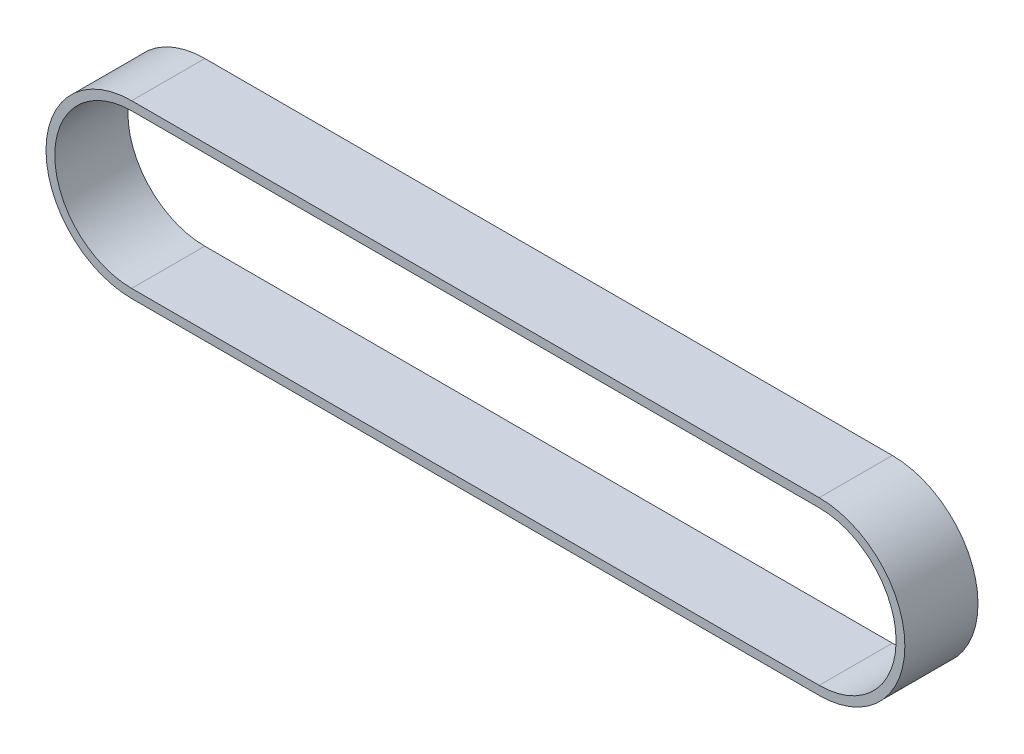
SolidWorks part; units mm, degrees
material "A6061"
ref_plane "Front Plane" through (0, 0, 0) normal (0, 0, 1) x (1, 0, 0)
ref_plane "Top Plane" through (0, 0, 0) normal (0, 1, 0) x (1, 0, 0)
ref_plane "Right Plane" through (0, 0, 0) normal (1, 0, 0) x (0, 0, -1)
sketch "Sketch2" plane through (0, 0, 0) normal (0, 0, 1) x (1, 0, 0)
  line L0 (0, 0) -> (1, 0) construction
  line L1 (0, 0) -> (0, 1) construction
  line L2 (0, -26.28) -> (-235, -26.28)
  line L3 (-235, 26.28) -> (0, 26.28)
  arc A0 (0, 26.28) -> (0, -26.28) centre (0, 0) cw
  arc A1 (-235, -26.28) -> (-235, 26.28) centre (-235, 0) cw
extrude "Extrude-Thin1" add sketch "Sketch2" along normal mid plane 25 thin thin type one direction wall 3
